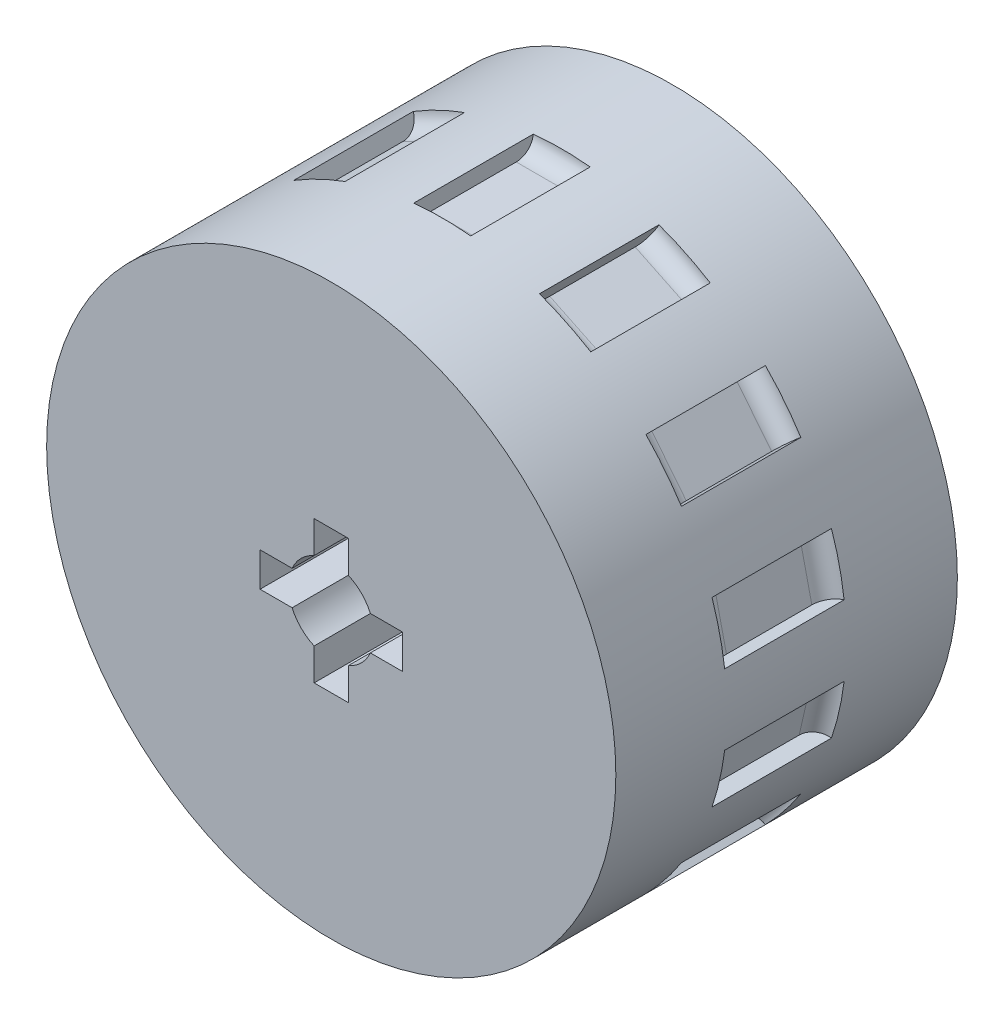
from build123d import *

# Parameters (mm, degrees)
SKETCH_1_R               = 50
EXTRUDE_1_DEPTH          = 60
EXTRUDE_START            = 5
SKETCH_2_R               = 13
SKETCH_2_R_2             = 7.5
EXTRUDE_1_2_DEPTH        = 5
CUT_EXTRUDE_1_DEPTH      = 5
PATTERN_CIRCULAR_1_COUNT = 14


with BuildPart() as part:
    # 草图1 → Extrude 1 (new body)
    with BuildSketch(Plane.XY):
        with Locations(Location((0, 0, 0), (0, 0, 180))):
            Circle(SKETCH_1_R)
        with BuildLine():
            Line((3, -6.873863542), (3, -12.5))
            Line((3, -12.5), (-3, -12.5))
            Line((-3, -12.5), (-3, -6.873863542))
            ThreePointArc((-3, -6.873863542), (-5.303300859, -5.303300859), (-6.873863542, -3))
            Line((-6.873863542, -3), (-12.5, -3))
            Line((-12.5, -3), (-12.5, 3))
            Line((-12.5, 3), (-6.873863542, 3))
            ThreePointArc((-6.873863542, 3), (-5.303300859, 5.303300859), (-3, 6.873863542))
            Line((-3, 6.873863542), (-3, 12.5))
            Line((-3, 12.5), (3, 12.5))
            Line((3, 12.5), (3, 6.873863542))
            ThreePointArc((3, 6.873863542), (5.303300859, 5.303300859), (6.873863542, 3))
            Line((6.873863542, 3), (12.5, 3))
            Line((12.5, 3), (12.5, -3))
            Line((12.5, -3), (6.873863542, -3))
            ThreePointArc((6.873863542, -3), (5.303300859, -5.303300859), (3, -6.873863542))
        make_face(mode=Mode.SUBTRACT)
    extrude(amount=EXTRUDE_1_DEPTH)

    # 草图2 → Extrude 1 2 (add)
    with BuildSketch(Plane(origin=(0, 0, 0), x_dir=(-1, 0, 0), z_dir=(0, 0, -1)).offset(EXTRUDE_START)):
        Circle(SKETCH_2_R)
        Circle(SKETCH_2_R_2, mode=Mode.SUBTRACT)
    extrude(amount=-EXTRUDE_1_2_DEPTH)

    # 草图3 → 切除-拉伸1 (cut, symmetric)
    with BuildSketch(Plane(origin=(0, 0, 0), x_dir=(0, 0, -1), z_dir=(1, 0, 0))):
        with BuildLine():
            Line((-37.5, 53), (-22.5, 53))
            ThreePointArc((-22.5, 53), (-19.5, 50), (-22.5, 47))
            Line((-22.5, 47), (-37.5, 47))
            ThreePointArc((-37.5, 47), (-40.5, 50), (-37.5, 53))
        make_face()
    cut_extrude_1 = extrude(amount=CUT_EXTRUDE_1_DEPTH, both=True, mode=Mode.SUBTRACT)

    # 阵列(圆周)1: 切除-拉伸1 ×14 about axis
    pattern_circular_1_axis = Axis((0, 0, 0), (0, 0, 1))
    for i in range(1, PATTERN_CIRCULAR_1_COUNT):
        add(cut_extrude_1.rotate(pattern_circular_1_axis, i * 360 / PATTERN_CIRCULAR_1_COUNT), mode=Mode.SUBTRACT)


solid = part.part
